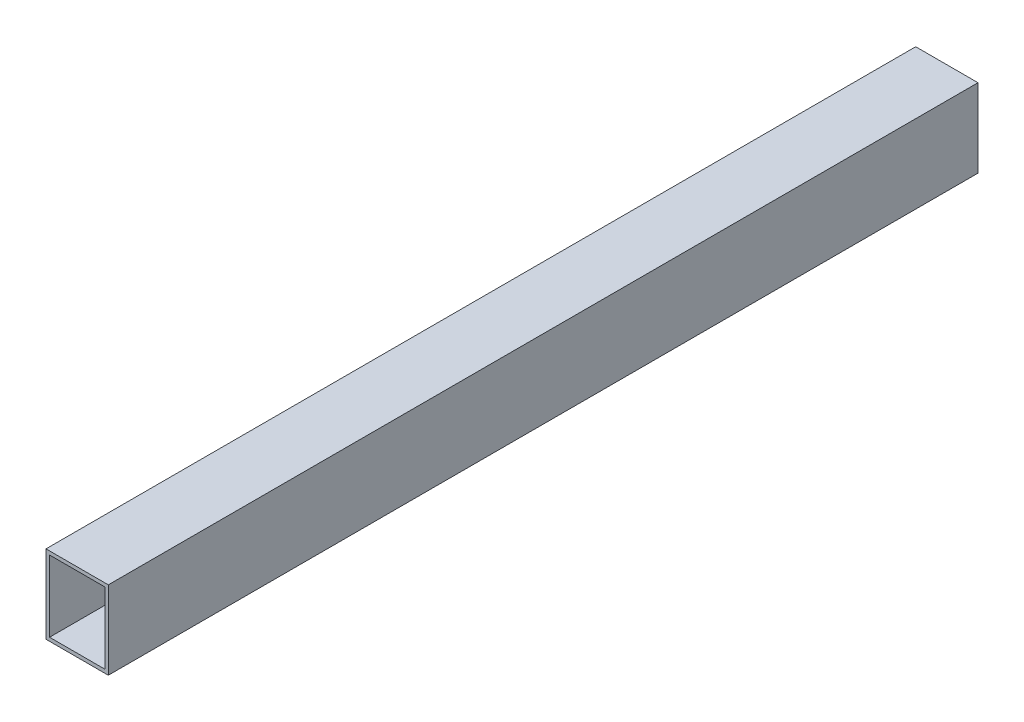
SolidWorks part; units mm, degrees
ref_plane "Front Plane" through (0, 0, 0) normal (0, 0, 1) x (1, 0, 0)
ref_plane "Top Plane" through (0, 0, 0) normal (0, 1, 0) x (1, 0, 0)
ref_plane "Right Plane" through (0, 0, 0) normal (1, 0, 0) x (0, 0, -1)
sketch "Sketch1" plane through (0, 0, 0) normal (0, 0, 1) x (1, 0, 0)
  line L0 (-15.5, 20) -> (15.5, 20)
  line L1 (-17.5, -22) -> (17.5, -22)
  line L2 (-17.5, -22) -> (-17.5, 22)
  line L3 (-17.5, 22) -> (17.5, 22)
  line L4 (17.5, -22) -> (17.5, 22)
  line L5 (-17.5, -22) -> (17.5, 22) construction
  line L6 (-17.5, 22) -> (17.5, -22) construction
  line L7 (15.5, -20) -> (15.5, 20)
  line L8 (-15.5, -20) -> (15.5, -20)
  line L9 (-15.5, -20) -> (-15.5, 20)
  point P0 (0, 0)
  dimension "D1" = 44
  dimension "D2" = 35
  dimension "D3" = 2
extrude "Boss-Extrude1" add sketch "Sketch1" along normal up to surface (488.4894 mm away)
